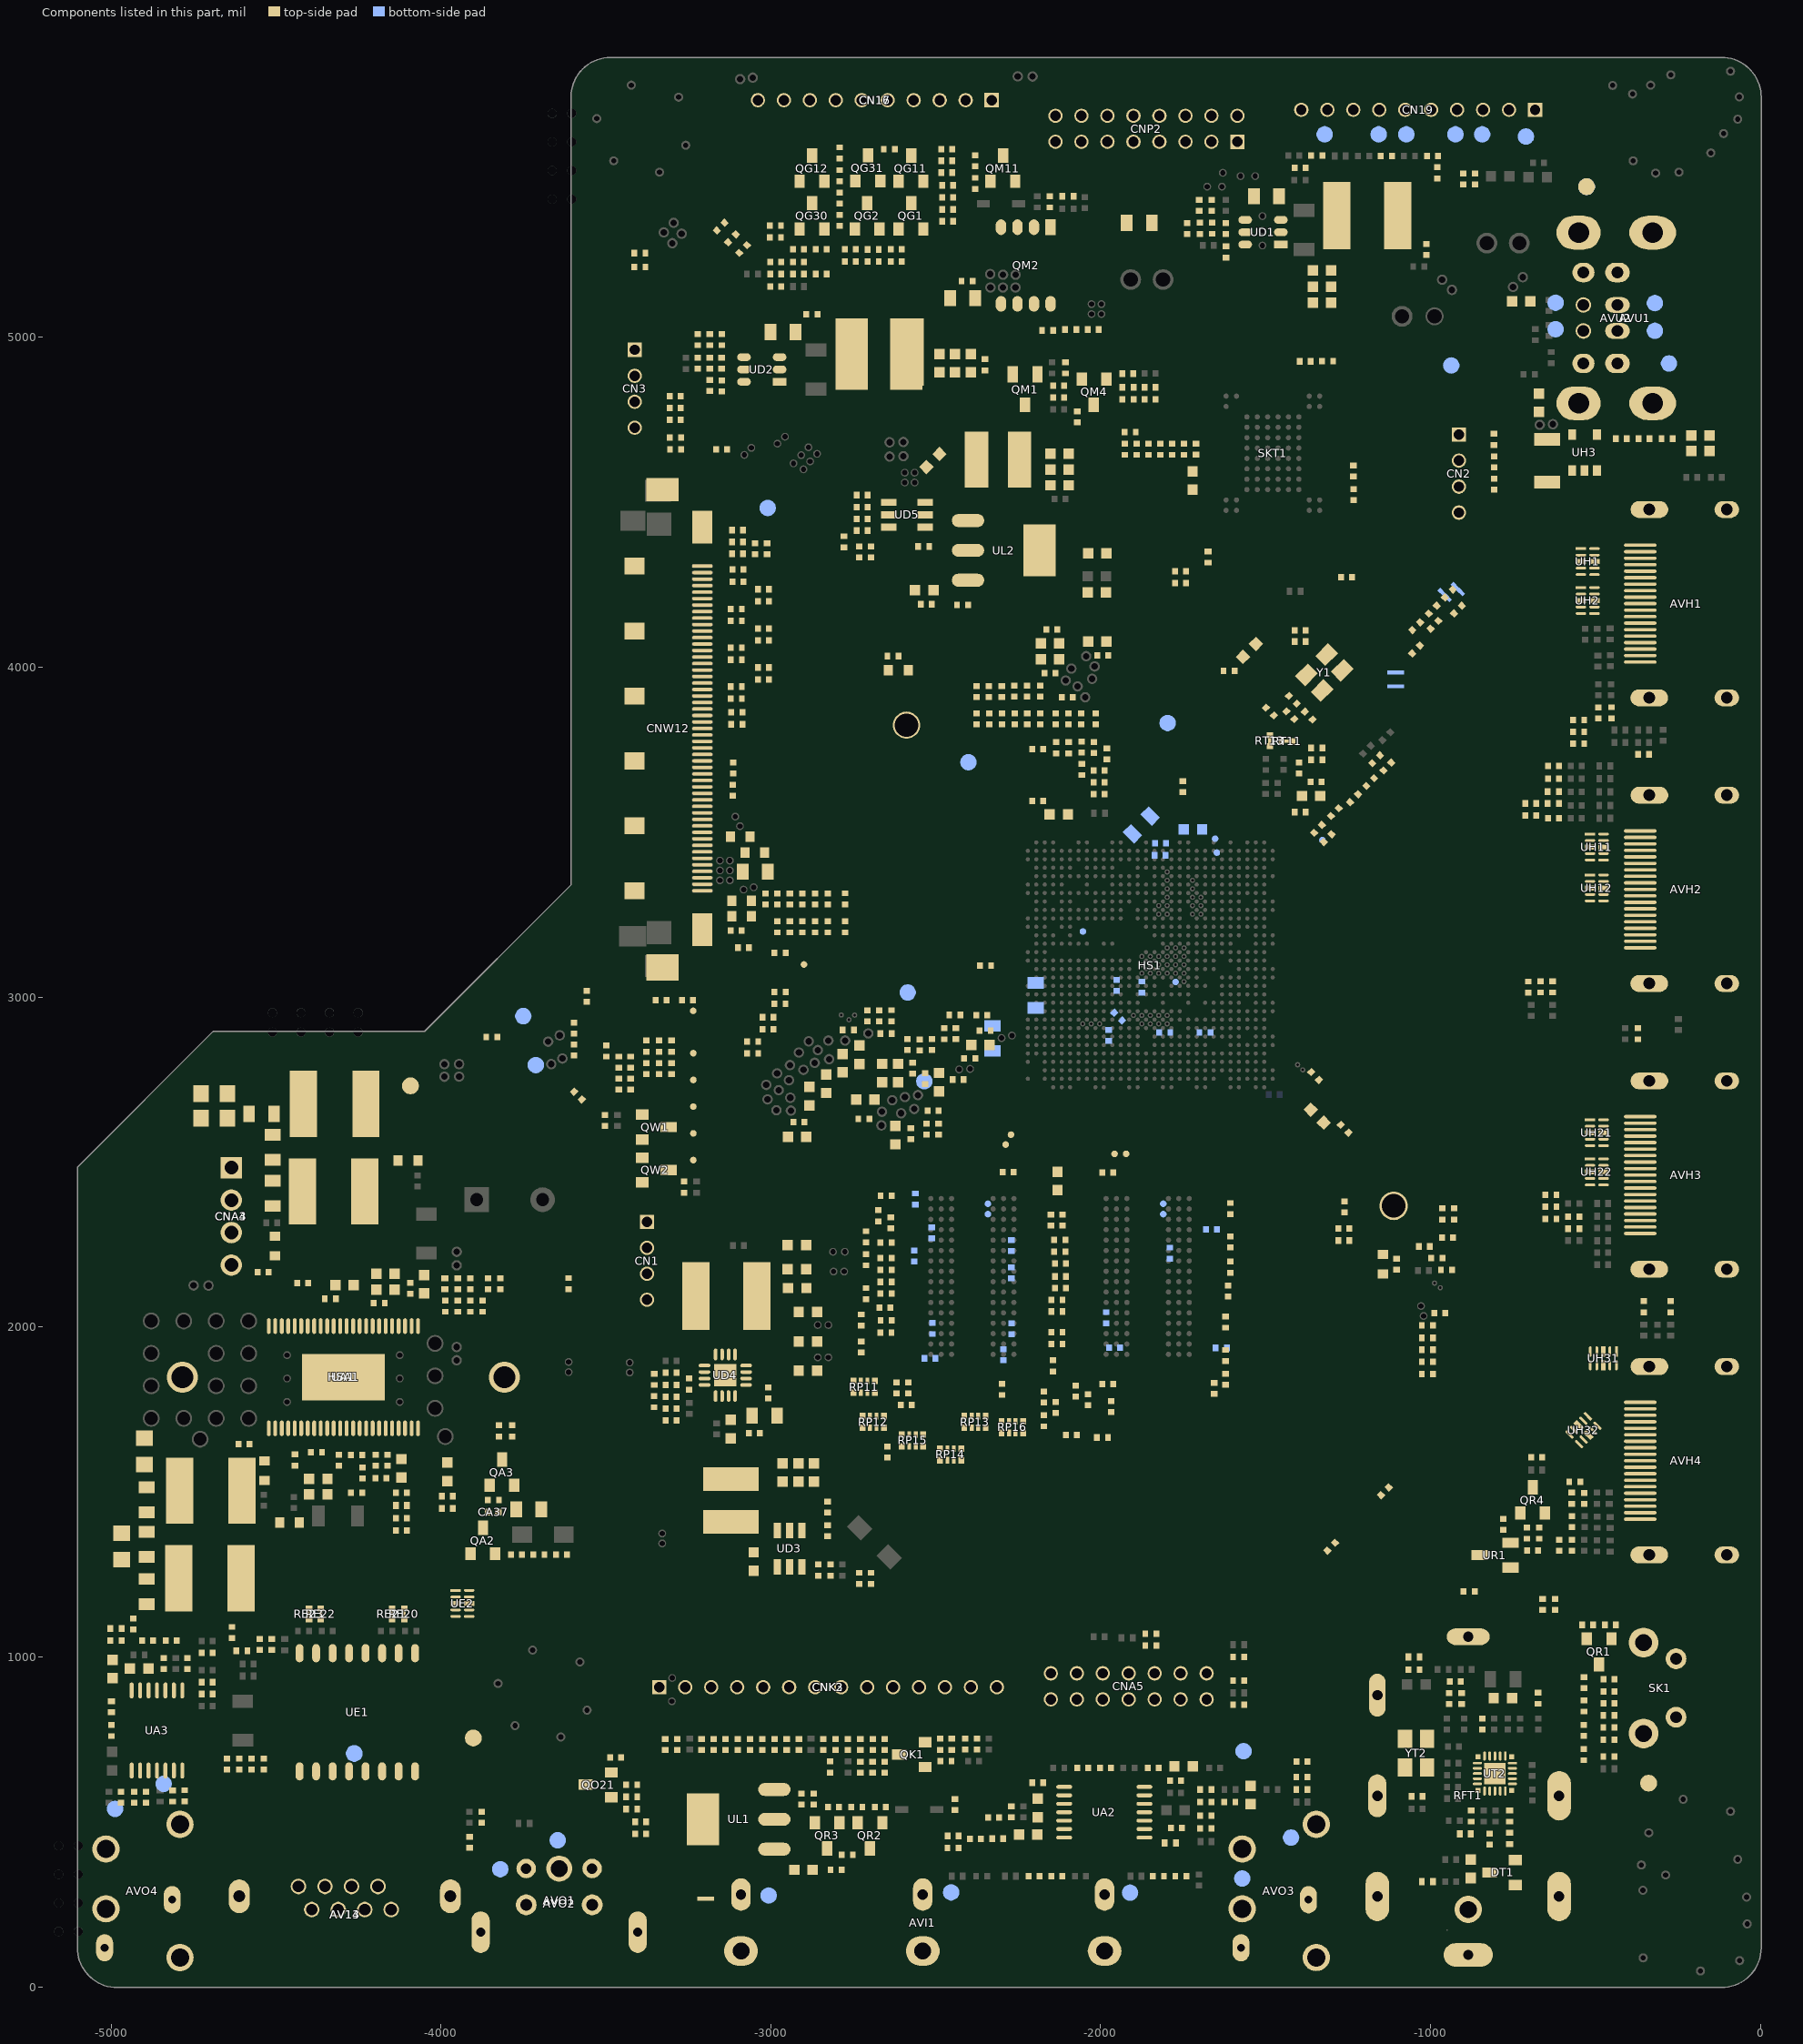
[diagram p0: the components of this part, seen from the top]
# Altium PCB MISC86290.PcbDoc (part 6 of 31)
Units mil, origin at the board's own origin, x right, y up, seen from the top; angles counter-clockwise.
Board outline 5104.71 x 5851.49 mil, 2 copper layers (TopLayer, BottomLayer), stack 61.855 mil thick; 1026 components, 667 nets, 4280 pads, 2294 vias.

## Footprints (in the part's own frame and the unit in brackets; to place one, negate y for a bottom-side part, rotate by r counter-clockwise, add the part's x,y. Pads: shape width x height; smd on the part's side, far side on the other; paste and mask are expansions set on the pad) (continued)
FFC51H/0.5SA-1 [mm] "FI-R E 51 S-HF,客户要求，与现库内1脚顺序相反"
  rect 0.25x1.55 smd: 1(-12.5,2.612)
  oval 0.25x1.55 smd: 2(-12,2.613) 3(-11.5,2.613) 4(-11,2.613) 5(-10.5,2.613) 6(-10,2.613) 7(-9.5,2.612) 8(-9,2.612) 9(-8.5,2.613) 10(-8,2.613) 11(-7.5,2.613) 12(-7,2.613) 13(-6.5,2.613) 14(-6,2.612) 15(-5.5,2.613) 16(-5,2.613) 17(-4.5,2.613) 18(-4,2.613) 19(-3.5,2.613) 20(-3,2.612) 21(-2.5,2.612) 22(-2,2.612) 23(-1.5,2.613) 24(-1,2.613) 25(-0.5,2.613) 26(0,2.613) 27(0.5,2.613) 28(1,2.612) 29(1.5,2.613) 30(2,2.613) 31(2.5,2.613) 32(3,2.613) 33(3.5,2.613) 34(4,2.613) 35(4.5,2.612) 36(5,2.612) 37(5.5,2.613) 38(6,2.613) 39(6.5,2.613) 40(7,2.613) 41(7.5,2.613) 42(8,2.612) 43(8.5,2.613) 44(9,2.613) 45(9.5,2.613) 46(10,2.613) 47(10.5,2.613) 48(11,2.612) 49(11.5,2.612) 50(12,2.613) 51(12.5,2.613)
  rect 2.5x1.55 smd: 52(-15.5,2.613) 60(15.5,2.612)
  rect 1.8x2.5 smd: 53(-18.4,-0.462)
  rect 1.3x1.55 smd: 54(-12.5,-2.612) 55(-7.5,-2.612) 56(-2.5,-2.612) 57(2.5,-2.612) 58(7.5,-2.612) 59(12.5,-2.612)
  rect 2.05x2.5 smd: 61(18.4,-0.462)
  silkscreen extent -18.25,-2.31 18.25,4.42
FUSE1.1A-S [mm] "保险丝：FSMD005-1206(FUZETEC)（兼容1206F8.00A063V 高度0.8mm），18.03.07）"
  rect 1x2 smd: 1(-1.65,0) 2(1.65,0)
  silkscreen extent -2.4,-1.2 2.4,1.2, body extent -1.75,-0.9 1.75,0.9, height 1
GND [mm] "导通线"
  rect 0.66x0.3 smd paste-0.45 mask-0.45: JP_1K(-0.32,0) JP_2K(0.32,0)
HDMI-HS-1 [mm] "浙江和丰   HHF-14B000-2SA。17.09.25更新钢网;171107更新焊盘露铜位置(18.04.19 更新大脚孔径）"
  rect 2.2x3.8 on Top Paste: 0(-7.75,4.18) 0(7.753,4.183)
  rect 2.2x6 on Top Paste: 0(-7.75,9.355) 0(7.75,9.355)
  oval 0.26x2.5 smd: 1(4.5,11.258) 2(4,11.258) 3(3.5,11.258) 4(3,11.258) 5(2.5,11.258) 6(2,11.258) 7(1.5,11.258) 8(1,11.258) 9(0.5,11.258) 10(0,11.258) 11(-0.5,11.258) 12(-1,11.258) 13(-1.5,11.258) 14(-2,11.258) 15(-2.5,11.258) 16(-3,11.258) 17(-3.5,11.258) 18(-4,11.258) 19(-4.5,11.258)
  oval 1.3x2.9 hole 0.9 slot 2.5 at 90 deg mask+0.076: 20(-7.25,10.565) 22(7.25,10.55)
  oval 1.3x1.9 hole 0.9 slot 1.5 at 90 deg mask+0.076: 21(-7.25,4.59) 23(7.25,4.59)
  silkscreen extent -7.5,2 7.5,12.19, body extent -10.25,-57.68 10.25,12.17, height 8.42
HS(27*10*10)-1 [mm] "同辉达，27*10*10"
  round 2.6 on Top Overlay: 0(0,12.4) 0(0,-12.4)
  round 2.4 hole 1.7: 1(0,12.4) 2(0,-12.4)
  silkscreen extent -5.1,-13.85 5.1,13.85
HS(55*55*10) [mm] "同辉达；55×55×10-黑色-THD(18.11.09 优化外框丝印）"
  round 3 on Top Overlay: 0(-18.45,-18.77) 0(18.56,18.74)
  round 2.1 / inner round 2.8 / far side round 2.8 hole 1.8: 1(-18.45,-18.77)
  round 2.2 / inner round 2.8 / far side round 2.8 hole 1.8: 2(18.56,18.74)
  silkscreen extent -27.65,-27.65 27.65,27.65
KEY-HD-6 [mm] "春生KFC-A06--E-4-160-7.5/4; 中心高度为4mm;14.09.04;171102修正突出距离"
  round 2.5 on Top Overlay: 0(-3.5,5) 0(3.5,5)
  round 1.8 on Top Overlay: 0(-2.25,2.5) 0(2.25,2.5)
  round 1.6 hole 0.9: 1(2.25,2.5) 2(-2.25,2.5)
  round 2.286 hole 1.3: 3(3.5,5) 4(-3.5,5)
  silkscreen extent -3.85,0 3.85,6.6
L0402 [mm]
  rect 0.45x0.55 smd mask+0.076: 1(-0.425,0) 2(0.425,0)
  silkscreen extent -0.8,-0.42 0.8,0.43, body extent -0.5,-0.25 0.5,0.25, height 0.5
L0603 [mil]
  rect 32x31.5 smd mask+3: 1(-27.81,0) 2(27.81,0)
  silkscreen extent -50,-22 50,22, body extent -31,-16 31,16, height 31
L0805 [mm] "片式磁珠、电感"
  rect 1.2x1.3 smd: 1(-1.016,0) 2(1.016,0)
  silkscreen extent -1.92,-0.95 1.92,0.95, body extent -1,-0.62 1,0.63, height 1.25
L(4.5*3.5)-S [mm] "SMD4532-6R8M-023"
  rect 1.8x4.3 smd: 1(-1.65,0) 2(1.65,0)
  TopLayer pour cut-out: -0.76,2.15 0.796,2.15 0.796,2.141 0.796,-2.149 -0.756,-2.149 -0.756,-2.15
  silkscreen extent -2.83,-2.44 3.3,2.44
L(5.8*4.5)-S [mm] "APC52A45M4R7\电感\Cailank;170317更新阻焊兼容L(4*3.0)-S"
  rect 2.5x5.5 smd paste-5.5: 1(2.105,0) 2(-2.105,0)
  TopLayer pour cut-out: -0.849,2.746 -0.845,2.75 0.861,2.75 0.861,-2.749 0.861,-2.753 0.859,-2.753 -0.862,-2.753
  silkscreen extent -1.5,-2.9 3.88,2.9, body extent -3.06,-2.65 3.08,2.74, height 4.8
L(6.0*4.5)-S#1 [mm]
  rect 2.1x5.1 smd paste-6: 1(-2.4,0) 2(2.4,0)
  TopLayer pour cut-out: -1.404,2.552 1.416,2.543 1.417,2.544 1.416,2.544 1.419,-2.546 -1.433,-2.549 -1.433,-2.544 -1.433,-2.543
  silkscreen extent -3,-3.1 3.95,3.1
L(6.0*4.5)-S#2 [mm] "SWPA6045S4R7MT(Sunlord) :功率电感;161103更新焊盘大小"
  rect 2.1x5.2 smd paste-6: 1(-2.35,0) 2(2.35,0)
  TopLayer pour cut-out: -1.282,2.552 1.294,2.543 1.297,-2.547 -1.311,-2.549
  silkscreen extent -3.16,-3.15 3.9,3.15, body extent -3,-3 3,3, height 4.5
Manufacture_Info [mm]
  round 0.3 on Mech2: 0(0,0)
MARK [mm] "SMD 使用"
  round 1.3 smd paste+0 mask+0.65: 0(0,0)
  TopLayer circle w0.254: c0,0 r1.444
  TopLayer pour cut-out: -1.3,0 -1.201,-0.497 -0.919,-0.919 -0.497,-1.201 0,-1.3 0,-1.3 0.497,-1.201 0.919,-0.919 1.201,-0.497 1.3,0 1.3,0 1.201,0.497 0.919,0.919 0.497,1.201 0,1.3 0,1.3 -0.497,1.201 -0.919,0.919 -1.201,0.497 -1.3,0
OPTICAL-HD-6 [mm] "DQ,DQT-015B1,17.05.11"
  round 2 on Keep-Out: 0(-2.802,4.65) 0(2.798,4.65)
  round 1.8 on Top Overlay: 0(-2.54,7.3) 0(2.54,7.3)
  round 1.7 on Top Overlay: 0(-2.54,10.1) 0(0,10.1) 0(2.54,10.1)
  round 1.5 hole 0.8: 1(-2.54,10.1) 2(0,10.1) 3(2.54,10.1)
  round 1.6 hole 0.9: 4(2.54,7.3) 5(-2.54,7.3)
  silkscreen extent -4.95,0 4.95,12.73, body extent -4.83,-1 4.82,12.5, height 10.05
PCB_NAME [mm]
  round 0.3 on Mech2: 0(0,0)
PCB_TIME [mm]
  round 0.3 on Mech2: 0(0,0)
PHONE-HD-42 [mm] "YUQIU;PJ7724-F05L3BE-D;160401(17.07.18,孔内边增加0.1mm，外距不变）(18.03.13 更新孔径）"
  oval 1.5x2.3 on Top Overlay: 0(-3,3) 8(2.2,6.7)
  round 2.3 on Top Overlay: 0(-2.9,6) 0(-2.9,10.6) 0(2.8,2.25) 0(2.8,12.5)
  round 2.1 hole 1.4: 1(2.8,2.25) 3(2.8,12.5) 4(-2.9,6) 5(-2.9,10.6)
  oval 1.3x2.1 hole 0.6 slot 1.4 at 90 deg: 2(-3,3) 6(2.2,6.7)
  silkscreen extent -3.65,0 3.65,13.15, body extent -5.05,-62.22 5.05,13, height 12.05
QFN16/0.5-4 [mm] "TI,TLV62095,17.11.08"
  oval 0.9x0.28 smd: 1(-1.6,0.75) 2(-1.6,0.25) 3(-1.6,-0.25) 4(-1.6,-0.75) 9(1.6,-0.75) 10(1.6,-0.25) 11(1.6,0.25) 12(1.6,0.75)
  oval 0.28x0.9 smd: 5(-0.75,-1.6) 6(-0.25,-1.6) 7(0.25,-1.6) 8(0.75,-1.6) 13(0.75,1.6) 14(0.25,1.6) 15(-0.25,1.6) 16(-0.75,1.6)
  rect 1.7x1.7 smd paste-0.7 mask-0.7: EPAD(0,0)
  silkscreen extent -2.86,-2.67 2.71,2.71, body extent -1.6,-1.6 1.6,1.6, height 1
QFN24/0.4-1 [mm]
  rect 0.4x0.4 smd: 1(-1.295,1.295) 7(-1.295,-1.295) 13(1.295,-1.295) 19(1.295,1.295)
  oval 0.7x0.2 smd: 2(-1.35,0.8) 3(-1.35,0.4) 4(-1.35,0) 6(-1.35,-0.8) 14(1.35,-0.8) 15(1.35,-0.4) 16(1.35,0) 17(1.35,0.4) 18(1.35,0.8)
  oval 0.7x0.2 smd paste+0: 5(-1.35,-0.4)
  oval 0.2x0.7 smd: 8(-0.8,-1.35) 9(-0.4,-1.35) 10(0,-1.35) 11(0.4,-1.35) 12(0.8,-1.35) 20(0.8,1.35) 21(0.4,1.35) 22(0,1.35) 23(-0.4,1.35)
  oval 0.2x0.7 smd paste+0: 24(-0.8,1.35)
  rect 1.651x1.651 smd paste-2 mask-2: EPAD(0,0)
  silkscreen extent -2.4,-2.24 2.11,2.7, body extent -1.5,-1.5 1.5,1.5, height 0.9
R0402 [mm] "片式电阻"
  rect 0.45x0.5 smd mask+0.076: 1(-0.425,0) 2(0.425,0)
  silkscreen extent -0.8,-0.4 0.8,0.4, body extent -0.5,-0.25 0.5,0.25, height 0.5
R0402SC [mm]
  rect 0.45x0.5 smd mask+0.076: 1(-0.425,0) 2(0.425,0)
  rect 0.42x0.25 smd paste-0.5 mask-0.5: 3(0,0)
  silkscreen extent -0.8,-0.4 0.8,0.4
R0603 [mm] "贴片电阻"
  rect 0.7x0.8 smd mask+0.076: 1(-0.756,0) 2(0.756,0)
  silkscreen extent -1.25,-0.54 1.25,0.54, body extent -0.8,-0.4 0.8,0.4, height 0.8
RA0402-MSD6886 [mm] "0402排阻  MSD6886方案DDR专用  满足DDR 5mil布线规则，18.08.22"
  rect 0.5x0.45 smd mask+0.076: 1(-0.45,0.825) 2(0.45,0.825) 7(-0.45,-0.825) 8(0.45,-0.825)
  rect 0.5x0.3 smd mask+0.076: 3(-0.45,0.25) 4(0.45,0.25) 5(-0.45,-0.25) 6(0.45,-0.25)
  silkscreen extent -0.85,-1.27 0.85,1.27, body extent -0.51,-1 0.51,1, height 0.35
RCL0524P [mm] "RCLAMP0524J"
  rect 0.21x0.8 smd: 1(-1,-0.52)
  oval 0.21x0.8 smd: 2(-0.5,-0.52) 3(0.5,-0.52) 4(1,-0.52) 5(1,0.52) 6(0.5,0.52) 7(-0.5,0.52) 8(-1,0.52)
  rect 0.38x0.8 smd: GND(0,0.52) GND(0,-0.52)
  silkscreen extent -1.4,-2.03 1.4,1.1, body extent -1.25,-0.6 1.25,0.6, height 0.66
RJ45U-D-5 [mm] "深圳普盈电子 规格：509053073，RJ45 8P8C 无灯无弹ROHS"
  oval 1.8x2.8 on Top Overlay: 0(-8.13,8.96) 0(8.13,8.96)
  round 3.25 on Keep-Out: 0(-6.35,5.4) 0(6.35,5.4)
  round 1.4 on Top Overlay: 0(-3.57,9.72) 0(-2.55,7.94) 0(-1.53,9.72) 0(-0.51,7.94) 0(0.51,9.72) 0(1.53,7.94) 0(2.55,9.72) 0(3.57,7.94)
  round 1.2 hole 0.9: 1(3.57,7.94) 2(2.55,9.72) 3(1.53,7.94) 4(0.51,9.72) 5(-0.51,7.94) 6(-1.53,9.72) 7(-2.55,7.94) 8(-3.57,9.72)
  oval 1.6x2.6 hole 0.9 slot 1.8 at 90 deg: 9(-8.13,8.96) 10(8.13,8.96)
  silkscreen extent -8.23,-0.04 8.23,15.75, body extent -8.29,0.1 8.29,16, height 13.1
RJ45U-D-14 [mm] "GLGNET：41238-01G051，无灯无弹片；170911"
  round 3.25 on Keep-Out: 0(-6.35,3.4) 0(6.35,3.4)
  round 1.2 hole 0.9: 1(3.57,5.94) 2(2.55,7.72) 3(1.53,5.94) 4(0.51,7.72) 5(-0.51,5.94) 6(-1.53,7.72) 7(-2.55,5.94) 8(-3.57,7.72)
  silkscreen extent -8,0 8.03,13.2, body extent -8.78,-61.25 8.72,13.3, height 15.64
SIP2*7/2.0D [mm] "捷仕泰"
  round 1.1 hole 0.8: 1(6,1) 2(6,-1) 3(4,1) 4(4,-1) 5(2,1) 6(2,-1) 7(0,1) 8(0,-1) 9(-2,1) 10(-2,-1) 11(-4,1) 12(-4,-1) 13(-6,1) 14(-6,-1)
  round 1.3 on Top Overlay: ""(-6,-1) ""(-6,1) ""(-4,1) ""(-4,-1) ""(-2,-1) ""(-2,1) ""(0,-1) ""(0,1) ""(2,-1) ""(2,1) ""(4,1) ""(4,-1) ""(6,-1)
  rect 1.3x1.3 on Top Overlay: ""(6,1)
  silkscreen extent -7.1,-3 7.85,3, body extent -7,-2.1 7,2.1, height 6
SIP2*8/2.0D-5 [mm] "捷仕泰；A2009A-209-A1MA-B,,插线高度11.5mm"
  round 1.3 on Top Overlay: 0(-7,-1) 0(-5,-1) 0(-5,1) 0(-3,-1) 0(-3,1) 0(-1,-1) 0(-1,1) 0(1,-1) 0(1,1) 0(3,-1) 0(3,1) 0(5,-1) 0(5,1) 0(7,-1) 0(7,1)
  rect 1.3x1.3 on Top Overlay: 0(-7,1)
  rect 1.1x1.1 hole 0.8: 1(-7,1)
  round 1.1 hole 0.8: 2(-7,-1) 3(-5,1) 4(-5,-1) 5(-3,1) 6(-3,-1) 7(-1,1) 8(-1,-1) 9(1,1) 10(1,-1) 11(3,1) 12(3,-1) 13(5,1) 14(5,-1) 15(7,1) 16(7,-1)
  silkscreen extent -9.54,-4.55 9.13,5.3
SIP4/2.0D-1 [mm] "捷仕泰/铭锋达"
  rect 1.6x1.6 on Top Overlay: 0(-3,0)
  round 1.6 on Top Overlay: 0(-1,0) 0(1,0) 0(3,0)
  rect 1.1x1.1 hole 0.8: 1(-3,0)
  round 1.1 hole 0.8: 2(-1,0) 3(1,0) 4(3,0)
  silkscreen extent -5.13,-3.2 5.12,1.8, body extent -5,-3.2 5,1.8, height 6
SIP4H/2.5D-4 [mm] "恩得利 4607-E04N-15B 带加强筋"
  rect 1.905x1.905 on Top Overlay: 0(-3.75,0)
  round 1.905 on Top Overlay: 0(-1.25,0) 0(1.25,0) 0(3.75,0)
  rect 1.651x1.651 hole 1.05: 1(-3.75,0)
  round 1.651 hole 1.05: 2(-1.25,0) 3(1.25,0) 4(3.75,0)
  silkscreen extent -6.26,-9.33 6.34,2.12
SIP4H/2.5D-7 [mm] "AMA,TJC3B-4AW,带扣、台阶。17.08.28"
  rect 1.85x1.85 on Top Overlay: 0(-3.75,0.18)
  round 1.85 on Top Overlay: 0(-1.25,0.18) 0(1.25,0.18) 0(3.75,0.18)
  rect 1.65x1.65 hole 1.05: 1(-3.75,0.18)
  round 1.65 hole 1.05: 2(-1.25,0.18) 3(1.25,0.18) 4(3.75,0.18)
  silkscreen extent -6.38,-7.35 6.38,1.91
SIP10/2.0D-1 [mm] "捷仕泰/铭锋达"
  rect 1.6x1.6 on Top Overlay: 0(-9,0)
  round 1.6 on Top Overlay: 0(-7,0) 0(-5,0) 0(-3,0) 0(-1,0) 0(1,0) 0(3,0) 0(5,0) 0(7,0) 0(9,0)
  rect 1.1x1.1 hole 0.8: 1(-9,0)
  round 1.1 hole 0.8: 2(-7,0) 3(-5,0) 4(-3,0) 5(-1,0) 6(1,0) 7(3,0) 8(5,0) 9(7,0) 10(9,0)
  silkscreen extent -11,-3.2 11,1.8, body extent -11,-3.2 11,1.8, height 6
SIP10/2.0D-4 [mm] "(HS)华琐电子  PHS-10A"
  rect 1.6x1.6 on Top Overlay: 0(-9,0)
  round 1.6 on Top Overlay: 0(-7,0) 0(-5,0) 0(-3,0) 0(-1,0) 0(1,0) 0(3,0) 0(5,0) 0(7,0) 0(9,0)
  rect 1.1x1.1 hole 0.8: 1(-9,0)
  round 1.1 hole 0.8: 2(-7,0) 3(-5,0) 4(-3,0) 5(-1,0) 6(1,0) 7(3,0) 8(5,0) 9(7,0) 10(9,0)
  silkscreen extent -11.1,-2.17 11.1,2.93, body extent -11.09,-2.17 11.09,2.93, height 8.1
SIP14/2.0D-2 [mm] "铭锋达/捷仕泰;K7改为NC 170224(17.06.29改小焊环，防止连锡）"
  rect 1.3x1.3 on Top Overlay: 0(-13,0)
  round 1.3 on Top Overlay: 0(-11,0) 0(-9,0) 0(-7,0) 0(-5,0) 0(-3,0) 0(-1,0) 0(1,0) 0(3,0) 0(5,0) 0(7,0) 0(9,0) 0(11,0) 0(13,0)
  rect 1.1x1.1 hole 0.8: 1(-13,0)
  round 1.1 hole 0.8: 2(-11,0) 3(-9,0) 4(-7,0) 5(-5,0) 6(-3,0) 7(-1,0) 8(1,0) 9(3,0) 10(5,0) 11(7,0) 12(9,0) 13(11,0) 14(13,0)
  silkscreen extent -15,-3.2 15,1.8, body extent -15,-3.2 15,1.8, height 6
SIP14/2.0D-5 [mm] "捷仕泰   A2004-14-A1MA-P,插线高度11mm"
  rect 1.3x1.3 on Top Overlay: 0(-13,0)
  round 1.3 on Top Overlay: 0(-11,0) 0(-9,0) 0(-7,0) 0(-5,0) 0(-3,0) 0(-1,0) 0(1,0) 0(3,0) 0(5,0) 0(7,0) 0(9,0) 0(11,0) 0(13,0)
  rect 1.1x1.1 hole 0.8: 1(-13,0)
  round 1.1 hole 0.8: 2(-11,0) 3(-9,0) 4(-7,0) 5(-5,0) 6(-3,0) 7(-1,0) 8(1,0) 9(3,0) 10(5,0) 11(7,0) 12(9,0) 13(11,0) 14(13,0)
  silkscreen extent -15,-2.13 15,3.07
SO-8 [mm] "AP2318(ULDO)"
  rect 1.2x0.8 smd: 1(-2.95,1.905)
  oval 1.2x0.8 smd: 2(-2.95,0.635) 3(-2.95,-0.635) 4(-2.95,-1.905) 5(2.95,-1.905) 6(2.95,-0.635) 7(2.95,0.635) 8(2.95,1.905)
  silkscreen extent -3.32,-2.54 2,3.61, body extent -3.1,-2.5 3.1,2.5, height 1.76
SO-23 [mm]
  rect 0.8x1 smd: 1(0.952,1.016) 3(-0.953,1.016)
  rect 0.8x1.1 smd: 2(0,-0.966)
  silkscreen extent -1.55,-0.86 1.55,0.36, body extent -1.5,-1.25 1.5,1.25, height 1.1
SOP6/0.95 [mm] "TEXAS-74lLC1G3157，MP1470GJ-Z 高度1.1mm"
  rect 1.05x0.6 smd: 1(-1.375,0.95)
  oval 1.05x0.6 smd: 2(-1.375,0) 3(-1.375,-0.95) 4(1.375,-0.95) 5(1.375,0) 6(1.375,0.95)
  silkscreen extent -2.15,-1.5 0.85,2.51, body extent -0.85,-1.5 0.85,1.5, height 1.45
SOP16/1.27-2 [mm] "Pulse, H1260NL H16101MC-C"
  oval 1.4x0.6 smd: 1(-4.55,4.445) 2(-4.55,3.175) 3(-4.55,1.905) 4(-4.55,0.635) 5(-4.55,-0.635) 6(-4.55,-1.905) 7(-4.55,-3.175) 8(-4.55,-4.445) 9(4.55,-4.445) 10(4.55,-3.175) 11(4.55,-1.905) 12(4.55,-0.635) 13(4.55,0.635) 14(4.55,1.905) 15(4.55,3.175) 16(4.55,4.445)
  silkscreen extent -6.2,-6.35 6.2,6.35, body extent -3.73,-6.35 3.72,6.35, height 6
SOP48/0.5-2 [mm] "TI; TAS5733LDCAR;160627"
  oval 1.2x0.3 smd mask+0.076: 1(-3.938,5.75) 2(-3.938,5.25) 3(-3.938,4.75) 4(-3.938,4.25) 5(-3.938,3.75) 6(-3.938,3.25) 7(-3.938,2.75) 8(-3.938,2.25) 9(-3.938,1.75) 10(-3.938,1.25) 11(-3.938,0.75) 12(-3.938,0.25) 13(-3.938,-0.25) 14(-3.938,-0.75) 15(-3.938,-1.25) 16(-3.938,-1.75) 17(-3.938,-2.25) 18(-3.938,-2.75) 19(-3.938,-3.25) 20(-3.938,-3.75) 21(-3.938,-4.25) 22(-3.938,-4.75) 23(-3.938,-5.25) 24(-3.938,-5.75) 25(3.938,-5.75) 26(3.938,-5.25) 27(3.938,-4.75) 28(3.938,-4.25) 29(3.938,-3.75) 30(3.938,-3.25) 31(3.938,-2.75) 32(3.938,-2.25) 33(3.938,-1.75) 34(3.938,-1.25) 35(3.938,-0.75) 36(3.938,-0.25) 37(3.938,0.25) 38(3.938,0.75) 39(3.938,1.25) 40(3.938,1.75) 41(3.938,2.25) 42(3.938,2.75) 43(3.938,3.25) 44(3.938,3.75) 45(3.938,4.25) 46(3.938,4.75) 47(3.938,5.25) 48(3.938,5.75)
  oct 1.6x2.7 on Top Paste mask+0.076: EPAD(-0.9,1.6) EPAD(-0.9,-1.6) EPAD(0.9,1.6) EPAD(0.9,-1.6)
  oct 1.6x2.7 on Top Solder mask+0.076: EPAD(-0.9,1.6) EPAD(-0.9,-1.6) EPAD(0.9,1.6) EPAD(0.9,-1.6)
  rect 3.6x6.4 smd paste-8.5 mask-8.5: EPAD(0,0)
  TopLayer lines w0.127: 0,5.4 0,3.2 ; -1.8,3.2 -1.8,4.342 -1.8,5.4 1.8,5.4 1.8,3.2 ; -1.8,-3.2 -1.8,-5.4 1.8,-5.4 1.8,-3.2 ; 0,-3.2 0,-5.4
  silkscreen extent -5.14,-6.3 5.14,6.51, body extent -3.1,-6.3 3.1,6.3, height 1.2
SOT-23 [mm]
  rect 0.8x1 smd: B(0.952,1.016) E(-0.953,1.016)
  rect 0.8x1.1 smd: C(-0.013,-0.966)
  silkscreen extent -1.55,-0.81 1.55,0.36, body extent -1.5,-1.25 1.5,1.25, height 1.1
SOT-23-1 [mm]
  rect 0.8x1.1 smd: D(0,-1.15)
  rect 0.8x1.27 smd: G(0.95,1.2) S(-0.95,1.2)
  TopLayer pour cut-out: -1.583,0.903 -1.583,-0.905 1.587,-0.905 1.587,0.903
  silkscreen extent -1.55,-1.05 1.55,0.33, body extent -1.52,-1.48 1.52,1.48, height 1.25
SOT-23-3-1 [mm] "LC1208;LC1208SPEC"
  rect 0.8x1.27 smd: 1(-0.95,-1.2) 2(0.95,-1.2) 3(0,1.2)
  silkscreen extent -1.54,0.32 1.55,1.05, body extent -1.52,-1.48 1.52,1.48, height 1.25
SOT-23-5 [mm] "LPW5206(1.295mm)"
  rect 0.6x0.8 smd: 1(-0.95,-1.375) 2(0,-1.375) 3(0.95,-1.375) 4(0.95,1.375) 5(-0.95,1.375)
  silkscreen extent -1.5,-2.49 1.5,0.85, body extent -1.5,-0.85 1.5,0.85, height 1.45
SOT-23-6 [mm] "RICHTEK RT9266//RT7295A(1mm)"
  rect 0.55x1.2 smd: 1(-0.95,-1.4) 2(0,-1.4) 3(0.95,-1.4) 4(0.95,1.4) 5(0,1.4) 6(-0.95,1.4)
  silkscreen extent -1.55,-3 1.55,0.9, body extent -1.55,-0.9 1.55,0.9, height 1.3
SOT-23-7 [mil] "对应2N7002 MOS管，大小和SOT-23一样"
  rect 31.5x50 smd: D(0,40)
  rect 31.5x39.37 smd: G(-37.5,-40) S(37.5,-40)
  TopLayer pour cut-out: 64.07,-39.32 64.07,36.28 -60.76,36.28 -60.76,-39.32
  silkscreen extent -60,-14 60,34, body extent -59,-49 59,49, height 43
SOT-223 [mm]
  oval 1x2.5 smd: 1(-2.3,-2.75) 2(0,-2.75) 3(2.3,-2.75)
  rect 4x2.5 smd: 4(0,2.75)
  TopLayer pour cut-out: 2.3,-1.188 2.3,-4.312 -2.345,-4.312 -2.64,-4.253 -2.891,-4.086 -3.058,-3.835 -3.117,-3.54 -3.117,-3.54 -2.299,-3.54 -2.299,-1.956 -3.124,-1.956 -3.066,-1.662 -2.899,-1.413 -2.65,-1.247 -2.356,-1.188 -2.356,-1.188
  silkscreen extent -3.45,-2.75 3.45,2.81, body extent -3.35,-3.3 3.35,3.4, height 1.7
SSOP14/0.65-1 [mm] "TI,MSP430G2001"
  oval 0.3x1.225 smd: 1(-1.95,-3.087) 2(-1.3,-3.087) 3(-0.65,-3.087) 4(0,-3.087) 5(0.65,-3.087) 6(1.3,-3.087) 7(1.95,-3.087) 8(1.95,3.087) 9(1.3,3.087) 10(0.65,3.087) 11(0,3.087) 12(-0.65,3.088) 13(-1.3,3.087) 14(-1.95,3.087)
  silkscreen extent -3.04,-4.35 2.55,4.6, body extent -2.55,-3.19 2.55,3.19, height 1.2
T-14.5×25×10-F14.5-2 [mm] "联鸿达；T-14.5×25×10-F14.5-LHD (一体); 中心出口高度6.3mm,20170121"
  oval 2.1x4.1 on Top Overlay: 0(-7,20) 0(-7,4.5) 0(-7,12.25) 0(7,12.25) 0(7,4.5)
  oval 4.1x2.1 on Top Overlay: 0(0,0) 0(0,24.5)
  round 2.3 on Top Overlay paste-2: 0(0,3.45)
  round 2.1 hole 1.3: 1(0,3.45)
  oval 3.8x1.8 hole 0.8 slot 2.8 at 0 deg: 2(0,-0.05)
  oval 1.8x3.8 hole 0.8 slot 2.8 at 90 deg: 3(-7,4.45) 7(7,12.2) 8(7,4.45)
  oval 1.397x3.302 / inner oval 1.8x3.8 / far side oval 1.8x3.8 hole 0.8 slot 2.8 at 90 deg: 4(-7,12.2)
  oval 1.27x3.302 / inner oval 1.8x3.8 / far side oval 1.8x3.8 hole 0.8 slot 2.8 at 90 deg: 5(-7,19.95)
  oval 3.302x1.27 / inner oval 3.8x1.8 / far side oval 3.8x1.8 hole 0.8 slot 2.8 at 0 deg: 6(0,24.45)
  KeepOutLayer pour cut-out: -1.438,3.45 -1.329,2.902 -1.019,2.438 -0.555,2.128 -0.007,2.019 -0.007,2.019 0.541,2.128 1.005,2.438 1.315,2.902 1.424,3.45 1.424,3.45 1.315,3.998 1.005,4.462 0.541,4.772 -0.007,4.881 -0.007,4.881 -0.555,4.772 -1.019,4.462 -1.329,3.998 -1.438,3.45
  silkscreen extent -8,-1.27 8,25.72
TEST-SG-BGA-6367 [mm] "SG-BGA-6367,测试座子"
  round 1.8 on Keep-Out: 1(6.863,-6.862) 3(6.863,6.863) 4(-6.862,6.863) 6(-6.862,-6.862)
  round 0.9 on Keep-Out: 2(6.863,4.323) 5(-6.863,-1.782)
  silkscreen extent -8.18,-8.18 8.18,8.18
TP [mil] "TEST POINT"
  round 50 smd paste-50: 1(0,0)
TP-20#1 [mil] "TEST POINT;0.5mm"
  round 20 smd paste-39.37: 1(0,0)
TP-20#2 [mil] "TEST POINT;0.5mm"
  round 20 smd: 1(0,0)
USB1-HD-2 [mm] "捷仕泰 ： U2504M-04-E1WD-C；170204加宽后壳丝印(18.03.12,更新信号脚孔径）"
  oval 2.7x3.9 on Top Overlay: 0(-6.57,10.257) 0(6.57,10.247)
  oval 1.7x2.1 on Top Overlay: 0(-3.5,12.957) 0(3.5,12.957)
  oval 1.5x1.9 hole 0.9 slot 1.4 at 90 deg: 1(-3.5,12.957) 4(3.5,12.957)
  oval 1.4x2.1 on Top Overlay: 1(-1,12.957) 2(1,12.957)
  oval 1.2x1.9 hole 0.9 slot 1.4 at 90 deg: 2(-1,12.957) 3(1,12.957)
  oval 2.4x3.6 / inner oval 2.4x3.6 / far side oval 2.8x4 hole 1.6 slot 2.3 at 90 deg: 5(6.57,10.247) 6(-6.57,10.247)
  TopLayer pour cut-out: 2.433,14.667 4.428,14.667 4.532,14.647 4.62,14.588 4.678,14.5 4.699,14.396 4.699,14.396 4.699,11.335 4.68,11.238 4.625,11.156 4.542,11.101 4.445,11.081 4.445,11.081 2.422,11.081 2.422,14.656
  KeepOutLayer pour cut-out: -3.49,14.696 -4.146,14.566 -4.703,14.194 -5.075,13.637 -5.206,12.98 -5.206,12.98 -5.206,12.94 -5.068,12.25 -4.677,11.665 -4.092,11.275 -3.402,11.137 -3.402,11.137 2.42,11.137 2.637,11.18 2.821,11.303 2.943,11.487 2.986,11.703 2.986,11.703 2.986,14.149 2.944,14.361 2.824,14.541 2.644,14.661 2.432,14.704 2.432,14.704 -3.482,14.704 -3.485,14.703 -3.487,14.701 -3.489,14.699 -3.49,14.696
  silkscreen extent -7.1,2.04 7.05,14.58, body extent -10,-87.25 10,14.14, height 8.2
USB2-HD-1 [mm] "双盟 DUAL USB A/F 90°,20170921修改宽度到15.2mm"
  oval 2.9x3.7 on Top Overlay: 0(-6.57,16) 0(-6.57,10.3) 0(6.57,16) 0(6.57,10.3)
  round 1.85 on Top Overlay: 0(-3.5,13.01) 0(-3.5,15.63) 0(3.5,13.01) 0(3.5,15.63)
  round 1.4 on Top Overlay: 0(-1,15.63) 0(-1,13.01) 0(1,15.63) 0(1,13.01)
  oval 1.5x1.7 hole 0.9: 1(-3.5,15.63) 4(3.5,15.63) 5(-3.5,13.01) 8(3.5,13.01)
  round 1.2 hole 0.9: 2(-1,15.63) 3(1,15.63) 6(-1,13.01) 7(1,13.01)
  oval 2.6x3.4 hole 1.6 slot 2.3 at 90 deg: 9(-6.57,16) 10(6.57,16) 11(-6.57,10.3) 12(6.57,10.3)
  KeepOutLayer pour cut-out: -5.206,13.033 -5.206,15.649 -4.578,15.021 -4.578,13.669 -5.214,13.033
  KeepOutLayer pour cut-out: -3.49,14.749 -4.146,14.618 -4.703,14.246 -5.075,13.69 -5.206,13.033 -5.206,13.033 -5.206,12.993 -5.068,12.303 -4.677,11.718 -4.092,11.327 -3.402,11.19 -3.402,11.19 2.42,11.19 2.637,11.233 2.821,11.356 2.943,11.539 2.986,11.756 2.986,11.756 2.986,14.202 2.944,14.414 2.824,14.594 2.644,14.714 2.432,14.756 2.432,14.756 -3.482,14.756 -3.485,14.756 -3.487,14.754 -3.489,14.752 -3.49,14.749
  KeepOutLayer pour cut-out: -3.49,17.369 -4.146,17.238 -4.703,16.866 -5.075,16.31 -5.206,15.653 -5.206,15.653 -5.206,15.613 -5.068,14.923 -4.677,14.338 -4.092,13.947 -3.402,13.81 -3.402,13.81 2.42,13.81 2.637,13.853 2.821,13.976 2.943,14.159 2.986,14.376 2.986,14.376 2.986,16.822 2.944,17.034 2.824,17.214 2.644,17.334 2.432,17.376 2.432,17.376 -3.482,17.376 -3.485,17.376 -3.487,17.374 -3.489,17.372 -3.49,17.369
  silkscreen extent -6.7,2 6.7,17.25, body extent -7.5,0 7.5,17, height 16.1
XTAL-S-3 [mm] "三星（SQ3D03200D2IBA）晶振"
  rect 1.4x1.1 smd: 1(-1.1,-0.85) 2(1.1,-0.85) 3(1.1,0.85) 4(-1.1,0.85)
  silkscreen extent -2.37,-1.9 1.65,1.3, body extent -1.65,-1.3 1.65,1.3, height 0.8

## Part data
AV13: library part XXX.XXX.0002342, "Network terminal,Network Terminal,DIP,5631-S-F-8C-1E-01,GLGNET-DLMI"
AV14: library part XXX.XXX.0002262, "Network terminal,Network Terminal,DIP,41238-01G051,GLGNET-DLMI"
AVH1 AVH2 AVH3 AVH4: library part 161011041-D-HDMI, "CN-HDMI-horizontal-#-#"
AVI1: library part "RCA端子,RCA Jack,AV3,H,Yellow、White、Red,CH5.5,D14,Seal,DIP,RC075-F03L3BY-A,YUQIU-DLMI-AV", "CN-AV-D14-#-#"
AVO1: library part "RCA端子,RCA Jack,AV1,H,Orange,CH5.5,Seal,DIP,AV38A-01S-5020,QS-DLMI"
AVO2: library part XXX.XXX.0002291, "Optical terminal,OPTICAL,H,DIP,DQT-015B1,DQ-DLMI"
AVO3 AVO4: library part XXX.XXX.0002138, "Earphone terminal,Earphone Jack,H,Φ3.5,CH7.0,Black,switch,Seal,DIP,PJ7724-F05L3BY-D,YUQIU-DLMI"
AVU1: library part USB-042M-002DP-DLMI-USB, "CN-USB-#-#-#"
AVU2: library part USB-A/F-90°-DLMI-USB, "CN-USB-double layer-#-#"
C1 C36 C61 C62 CD27 CD56: library part 004.003.0000671-D, "Ceramic capacitor,CAP MC,6.3V,22uF,±20%,X5R,0603,SMD,TP-D"
C2 C3 C4 C8 C12 C16 C19 C21 C25 C35 C39 C40 C41 C44 C51 C63 C64 C240 CD8 CD9 CD10 CD17 CD18 CD19 CD21 CD25 CD26 CD38 CD40 CD41 CD42 CD43 CD51 CD54 CD55 CF3 CL2 CL13 CO5 CO13 CO14: library part 004.003.0000383-D, "Ceramic capacitor,CAP MC,6.3V,10uF,±20%,X5R,0603,SMD,TP-D"
C5 C6 C7 C9 C13 C14 C15 C17 C18 C20 C22 C23 C24 C26 C27 C28 C29 C32 C33 C34 C38 C42 C43 C45 C110 C206 C207 C209 C210 C212 C213 CA9 CA15 CA20 CA23 CD4 CD12 CD14 CD16 CD22 CD29 CD30 CD52 CE6 CE7 CL1 CL3 CL25 CL55 CO1 CO21 CO24 CO25 CO37 CR2 CR3 CR4 CT31 CT33 CU1 CW244 CW245 CW246 CW247 CW248 CW249 CW250 CW251 CW252 CW253 CW254 CW255 CW256 CW257 CW258 CW259: library part 0.1uF-0402-X5R-±20%-16V-D
C10 C11 C30 C111: library part 004.003.0000100-D, "Ceramic capacitor,CAP MC,6.3V,2.2uF,±20%,X5R,0402,SMD,TP-D"
C37 CA10 CA16 CA21 CO17 CO19 CO35 CO41 CT30 CU2 CU3 CU5: library part 10uF-0603-X5R-±20%-6.3V-D
C46 C47 C48 C49 C50: library part 004.003.0000361-D, "Ceramic capacitor,CAP MC,6.3V,0.47uF,±10%,X5R,0402,SMD,TP-D"
C55: library part 004.003.0000562-D, "Ceramic capacitor,CAP MC,16V,0.047uF,±10%,X7R,0402,SMD,TP-D"
C56 C57 CO3: library part 33pF-0402-NPO-±5%-50V-D
C58 C60 C65 C66 C67 C68 C69 C70 C71 C73 C74 C75 C76 C77 C78 C79 C80 C81 C82 C83 C84 C85 C86 C87 C88 C89 C90 C91 C92 C93 C94 C95 C96 C97 C102 C103: library part 004.003.0000403-D, "Ceramic capacitor,CAP MC,16V,0.1uF,±20%,X5R,0402,SMD,TP-D"
C59 C98 C99 C100 C101 CA2 CA8 CA29 CO51 CO52: library part 004.003.0000503-D, "Ceramic capacitor,CAP MC,50V,1000pF,±10%,X7R,0402,SMD,TP-D"
C164: library part 2200pF-0402-X7R-±10%-50V-D
C174 CF1 CF2 CO4: library part 004.003.0000505-D, "Ceramic capacitor,CAP MC,16V,0.01uF,±10%,X7R,0402,SMD,TP-D"
C200 C201 RW52 RW53 RW55 RW56: library part 0ohm-0603-±5%-1/10W-D
C202 C205 CA37 CG1 CG11 CG30 CO33 CO34 CR1: library part 1uF-0402-X5R-±20%-6.3V-D
C208 C211 C214 CA36 CD3 CD11 CD33 CM17 CM18 CP1: library part 10uF-0805-X5R-±20%-16V-D
CA1 CA6: library part 004.003.0000044-D, "Ceramic capacitor,CAP MC,50V,0.1uF,±10%,X7R,0603,SMD,TP-D"
CA3 CA7: library part 4700pF-0402-X7R-±10%-50V-D
CA4 CA12 CA25: library part 004.003.0000667-D, "Ceramic capacitor,CAP MC,50V,1uF,±10%,X5R,0603,SMD,TP-D"
CA5 CA11 CA38 CA39 CI2 CT13: library part 0.047uF-0402-X7R-±10%-16V-D
CA13 CA19 CA22 CA28 CD35 CK3 CK9 CR5: library part 0.01uF-0402-X7R-±10%-50V-D
CA14 CA17 CA26 CA27: library part 0.68uF-0805-X7R-±10%-25V-D
CA18 CA24: library part 0.47uF-0805-X7R-±10%-50V-D